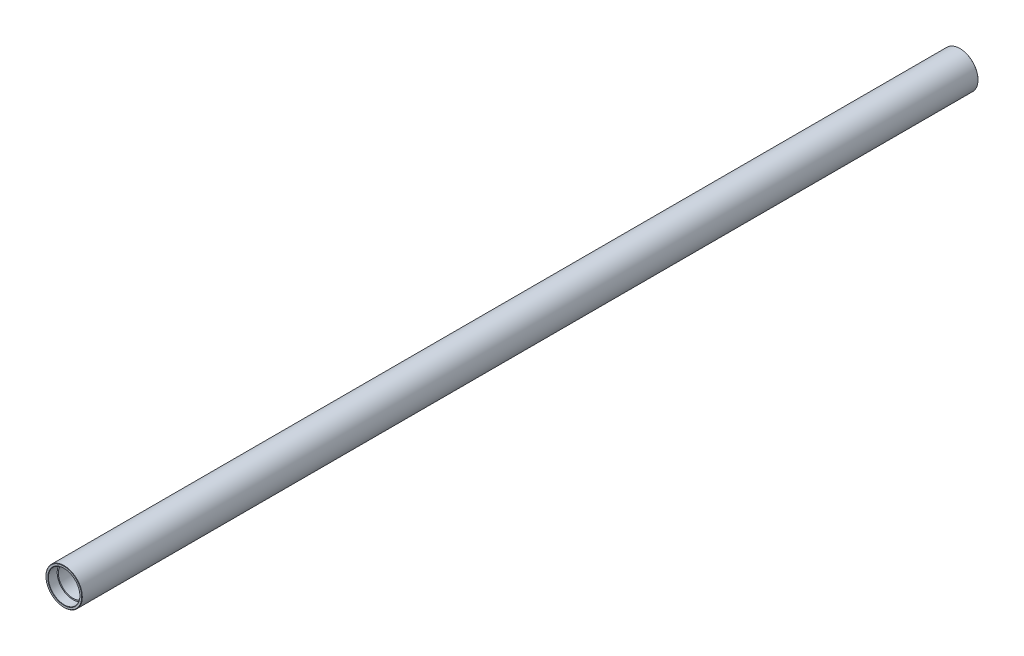
SolidWorks part; units mm, degrees
ref_plane "前视基准面" through (0, 0, 0) normal (0, 0, 1) x (1, 0, 0)
ref_plane "上视基准面" through (0, 0, 0) normal (0, 1, 0) x (1, 0, 0)
ref_plane "右视基准面" through (0, 0, 0) normal (1, 0, 0) x (0, 0, -1)
sketch "草图1" plane through (0, 0, 0) normal (0, 0, 1) x (1, 0, 0)
  circle A0 centre (0, 0) radius 30
  dimension "D1" = 60
extrude "凸台-拉伸1" add sketch "草图1" along normal blind 1480
sketch "草图2" plane through (0, 0, 0) normal (0, 0, -1) x (-1, 0, 0)
  circle A0 centre (0, 0) radius 24
  dimension "D1" = 48
extrude "切除-拉伸1" cut sketch "草图2" against normal blind 1600
sketch "草图3" plane through (0, 0, 0) normal (0, 0, -1) x (-1, 0, 0)
  circle A0 centre (0, 0) radius 26
  dimension "D1" = 52
extrude "切除-拉伸2" cut sketch "草图3" against normal blind 15
sketch "草图4" plane through (0, 0, 1480) normal (0, 0, 1) x (1, 0, 0)
  circle A0 centre (0, 0) radius 26
  dimension "D1" = 52
extrude "切除-拉伸3" cut sketch "草图4" against normal blind 15
chamfer "倒角1" distance 0.5 angle 45 4 edges at (-26, 0, 0) (30, 0, 0) (26, 0, 1480) (30, 0, 1480)
